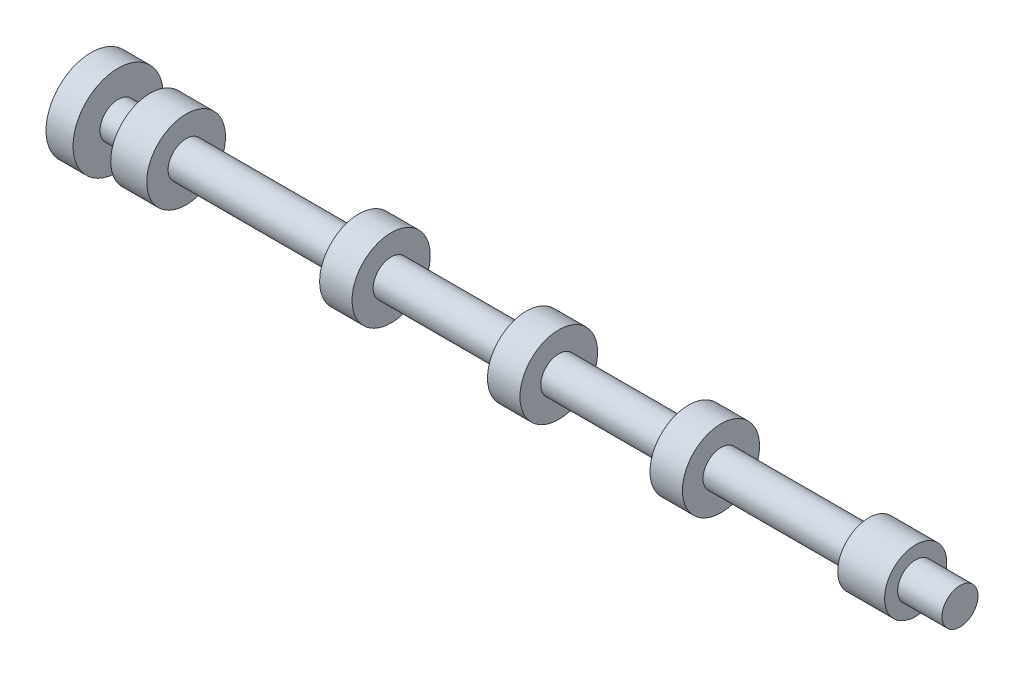
from build123d import *


with BuildPart() as part:
    # Sketch1 → Revolve1 (revolve)
    with BuildSketch(Plane.XY, mode=Mode.PRIVATE) as revolve1_sk:
        Polygon((-2966.670374904, 0), (-2484.570374904, 0), (-2484.570374904, 10), (-2509.170378936, 10), (-2509.170378936, 17.25), (-2535.170378936, 17.25), (-2535.170378936, 10), (-2617.170378936, 10), (-2617.170378936, 21.4), (-2635.170378936, 21.4), (-2635.170378936, 10), (-2707.170253936, 10), (-2707.170253936, 21.55), (-2725.170253936, 21.55), (-2725.170253936, 10), (-2800.170132968, 10), (-2800.170132968, 21.7), (-2818.170132968, 21.7), (-2818.170132968, 10), (-2913.920034929, 10), (-2913.920034929, 21.85), (-2933.920034929, 21.85), (-2933.920034929, 10), (-2951.670374904, 10), (-2951.670374904, 25), (-2966.670374904, 25), align=None)
    revolve(revolve1_sk.sketch.rotate(Axis((-2966.670374904, 0, 0), (1, 0, 0)), 90), axis=Axis((-2966.670374904, 0, 0), (1, 0, 0)))


solid = part.part
